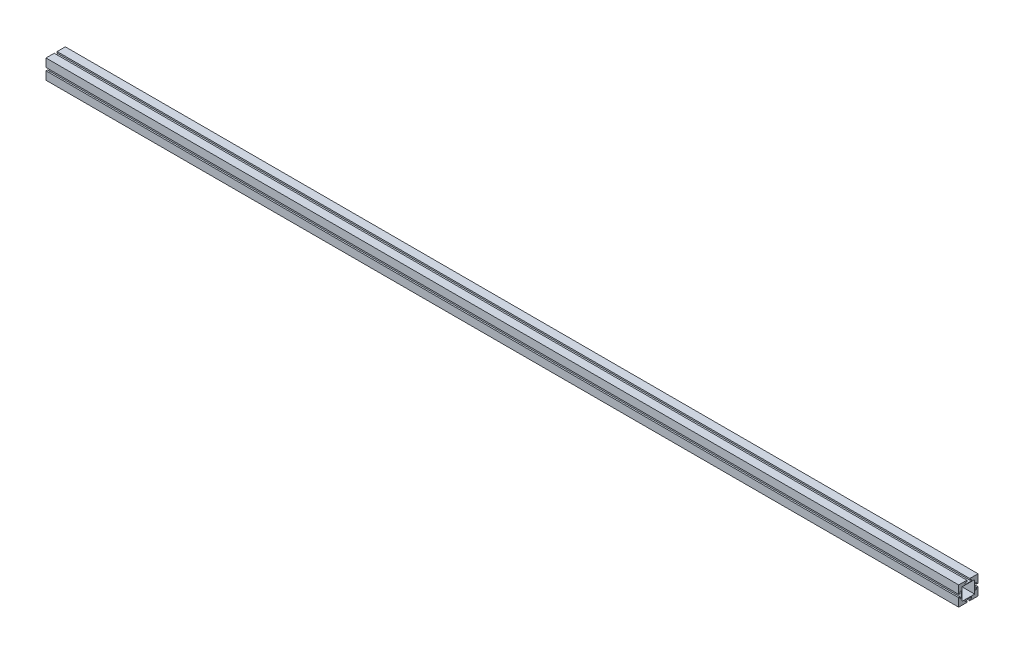
SolidWorks part; units mm, degrees
ref_plane "Front Plane" through (0, 0, 0) normal (0, 0, 1) x (1, 0, 0)
ref_plane "Top Plane" through (0, 0, 0) normal (0, 1, 0) x (1, 0, 0)
ref_plane "Right Plane" through (0, 0, 0) normal (1, 0, 0) x (0, 0, -1)
sketch "Sketch1" plane through (0, 0, 0) normal (1, 0, 0) x (0, 0, -1)
  line L0 (0, 0) -> (0, 33.8923) construction
  line L1 (-20, -20) -> (-3, -20)
  line L2 (-20, -20) -> (-20, -3)
  line L3 (-20, 20) -> (-3, 20)
  line L4 (20, -20) -> (20, -3)
  line L5 (-20, -20) -> (20, 20) construction
  line L6 (-20, 20) -> (20, -20) construction
  line L7 (-13, -13) -> (13, -13)
  line L8 (-13, -13) -> (-13, 13)
  line L9 (-13, 13) -> (13, 13)
  line L10 (13, -13) -> (13, 13)
  line L11 (-13, -13) -> (13, 13) construction
  line L12 (-13, 13) -> (13, -13) construction
  line L13 (0, 0) -> (25.505, 0) construction
  line L14 (17, 3) -> (17, 6.5)
  line L15 (-6.5, 17) -> (-3, 17)
  line L16 (6.5, 17) -> (6.5, 14)
  line L17 (3, 17) -> (6.5, 17)
  line L18 (-6.5, 14) -> (6.5, 14)
  line L19 (17, -6.5) -> (17, -3)
  line L20 (3, 20) -> (20, 20)
  line L21 (14, -6.5) -> (17, -6.5)
  line L22 (-3, 20) -> (-3, 17)
  line L23 (17, 3) -> (20, 3)
  line L24 (3, 20) -> (3, 17)
  line L25 (17, -3) -> (20, -3)
  line L26 (-20, 20) -> (20, 20) construction
  line L27 (14, -6.5) -> (14, 6.5)
  line L28 (-17, -17) -> (17, -17) construction
  line L29 (20, 3) -> (20, 20)
  line L30 (-6.5, 17) -> (-6.5, 14)
  line L31 (14, 6.5) -> (17, 6.5)
  line L32 (14, -14) -> (14, 14) construction
  line L33 (-14, 14) -> (14, 14) construction
  line L34 (-17, 17) -> (17, 17) construction
  line L35 (3, -20) -> (3, -17)
  line L36 (-17, -17) -> (-17, 17) construction
  line L37 (-14, -14) -> (-14, 14) construction
  line L38 (-14, -14) -> (14, -14) construction
  line L39 (17, -17) -> (17, 17) construction
  line L40 (20, -20) -> (20, 20) construction
  line L41 (3, -17) -> (6.5, -17)
  line L42 (6.5, -17) -> (6.5, -14)
  line L43 (-6.5, -14) -> (6.5, -14)
  line L44 (-6.5, -17) -> (-6.5, -14)
  line L45 (-6.5, -17) -> (-3, -17)
  line L46 (-3, -20) -> (-3, -17)
  line L47 (-14, -6.5) -> (-14, 6.5)
  line L48 (-14, -6.5) -> (-17, -6.5)
  line L49 (-17, -6.5) -> (-17, -3)
  line L50 (-17, -3) -> (-20, -3)
  line L51 (-17, 3) -> (-20, 3)
  line L52 (-17, 3) -> (-17, 6.5)
  line L53 (-14, 6.5) -> (-17, 6.5)
  line L54 (-20, 3) -> (-20, 20)
  line L55 (3, -20) -> (20, -20)
  line L56 (-20, -20) -> (-20, 20) construction
  line L58 (-20, -20) -> (20, -20) construction
  point P0 (0, 0)
  point P6 (0, 0)
  dimension "D1" = 40
  dimension "D2" = 40
  dimension "D3" = 26
  dimension "D4" = 26
  dimension "D7" = 3
  dimension "D8" = 3
  dimension "D9" = 6
  dimension "D10" = 13
  dimension "D11" = 3
  dimension "D12" = 6
  dimension "D13" = 13
  dimension "D5" = 3
  dimension "D6" = 3
extrude "Boss-Extrude1" add sketch "Sketch1" along normal blind 1890
